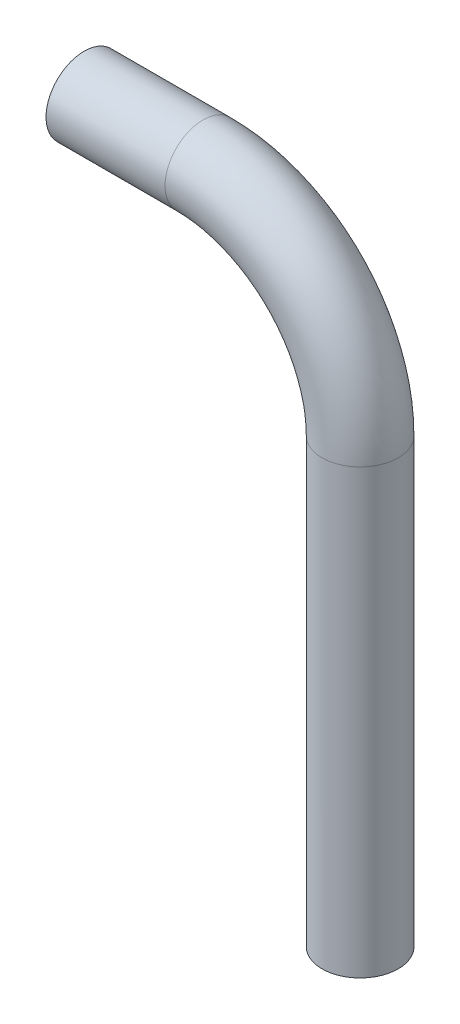
SolidWorks part; units mm, degrees
ref_plane "Front Plane" through (0, 0, 0) normal (0, 0, 1) x (1, 0, 0)
ref_plane "Top Plane" through (0, 0, 0) normal (0, 1, 0) x (1, 0, 0)
ref_plane "Right Plane" through (0, 0, 0) normal (1, 0, 0) x (0, 0, -1)
sketch "Sketch1" plane through (0, 0, 0) normal (0, 0, 1) x (1, 0, 0)
  line L0 (0, 0) -> (12.5, 0)
  line L1 (29, -16.5) -> (29, -63)
  arc A0 (12.5, 0) -> (29, -16.5) centre (12.5, -16.5) cw
  dimension "D1" = 16.5
sketch "Sketch2" plane through (0, 0, 0) normal (1, 0, 0) x (0, 0, -1)
  circle A0 centre (0, 0) radius 4
sweep "Sweep1" add profiles "Sketch2" path "Sketch1"
